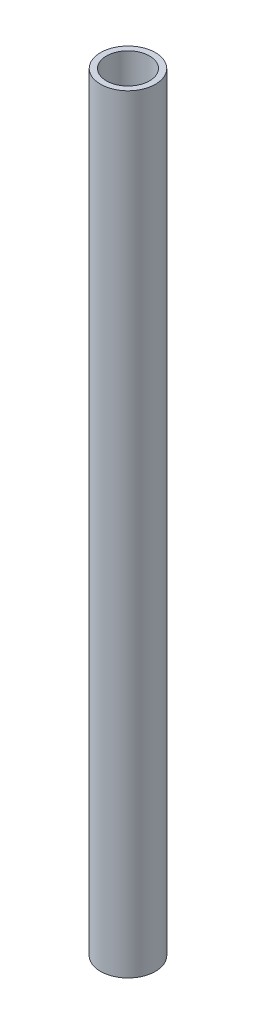
from build123d import *

# Parameters (mm, degrees)
SKETCH1_R           = 15
SKETCH1_R_2         = 11.8
BOSS_EXTRUDE1_DEPTH = 210


with BuildPart() as part:
    # Sketch1 → Boss-Extrude1 (new, symmetric)
    with BuildSketch(Plane(origin=(0, 0, 0), x_dir=(1, 0, 0), z_dir=(0, 1, 0))):
        with Locations(Location((0, 0, 0), (0, 0, 270))):
            Circle(SKETCH1_R)
        with Locations(Location((0, 0, 0), (0, 0, 270))):
            Circle(SKETCH1_R_2, mode=Mode.SUBTRACT)
    extrude(amount=BOSS_EXTRUDE1_DEPTH, both=True)


solid = part.part
